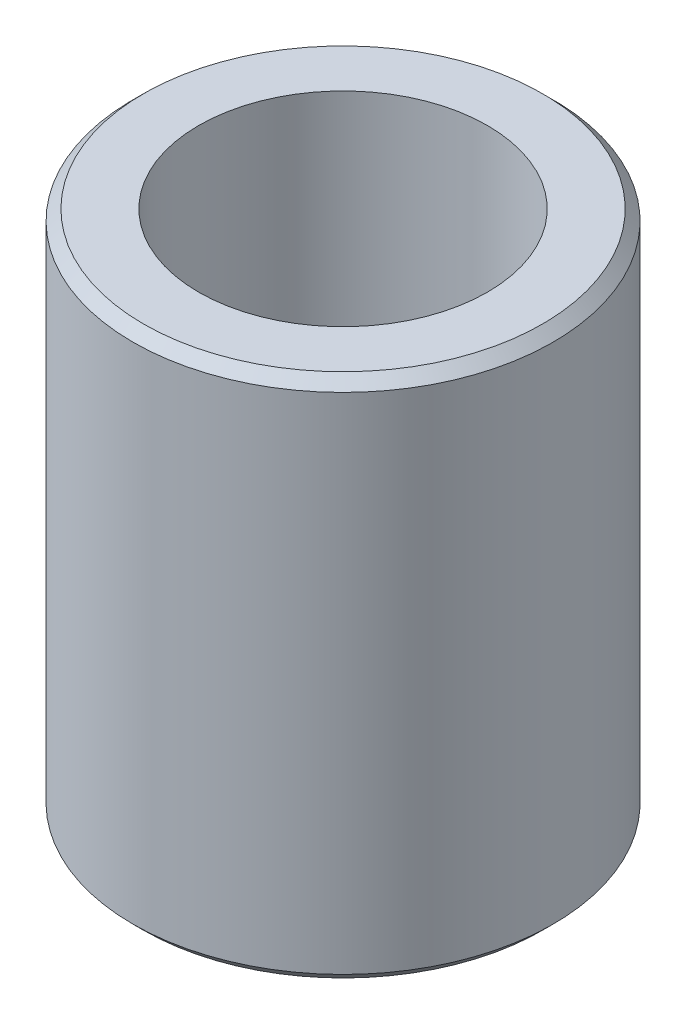
from build123d import *

# Parameters (mm, degrees)
SKETCH1_R           = 4
SKETCH1_R_2         = 2.75
BOSS_EXTRUDE1_DEPTH = 10
CHAMFER1_SIZE       = 0.2


with BuildPart() as part:
    # Sketch1 → Boss-Extrude1 (new body)
    with BuildSketch(Plane(origin=(0, 0, 0), x_dir=(1, 0, 0), z_dir=(0, 1, 0))):
        with Locations(Location((0, 0, 0), (0, 0, 270))):
            Circle(SKETCH1_R)
        with Locations(Location((0, 0, 0), (0, 0, 270))):
            Circle(SKETCH1_R_2, mode=Mode.SUBTRACT)
    extrude(amount=BOSS_EXTRUDE1_DEPTH)

    # Chamfer1
    chamfer1_edges = [part.edges().sort_by_distance(p)[0] for p in [
        (0, 0, -4),
        (0, 10, -4),
    ]]
    chamfer(chamfer1_edges, length=CHAMFER1_SIZE)


solid = part.part
